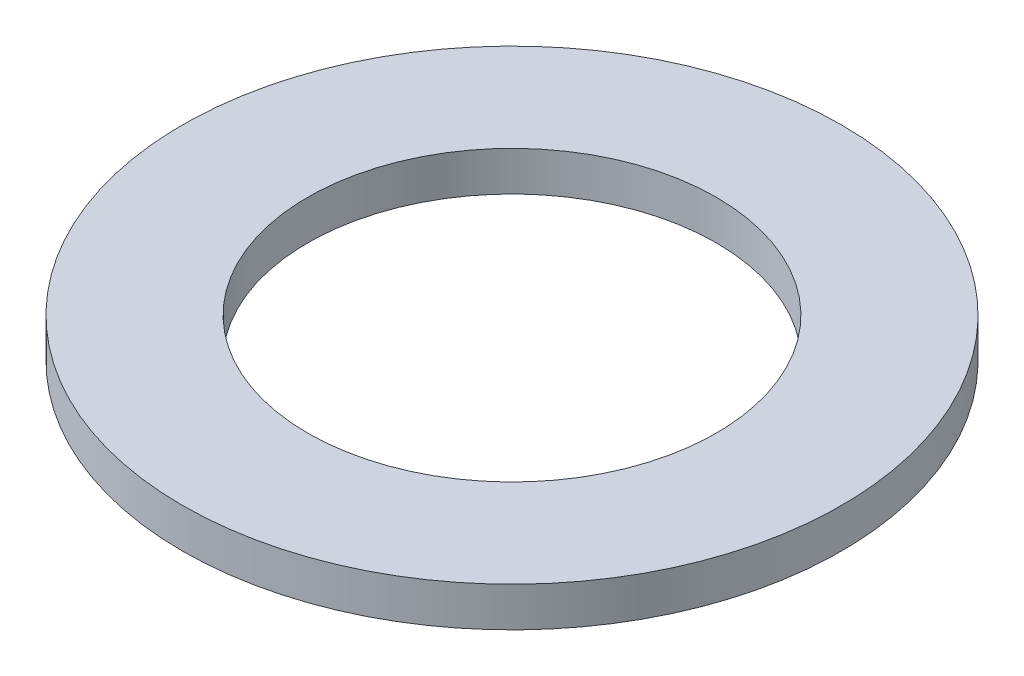
from build123d import *

# Parameters (mm, degrees)
SKETCH_1_R      = 25
SKETCH_1_R_2    = 15.5
EXTRUDE_1_DEPTH = 1.5


with BuildPart() as part:
    # 草图1 → 凸台-拉伸1 (new, symmetric)
    with BuildSketch(Plane(origin=(0, 0, 0), x_dir=(1, 0, 0), z_dir=(0, 1, 0))):
        with Locations(Location((0, 0, 0), (0, 0, 270))):
            Circle(SKETCH_1_R)
        with Locations(Location((0, 0, 0), (0, 0, 270))):
            Circle(SKETCH_1_R_2, mode=Mode.SUBTRACT)
    extrude(amount=EXTRUDE_1_DEPTH, both=True)


solid = part.part
